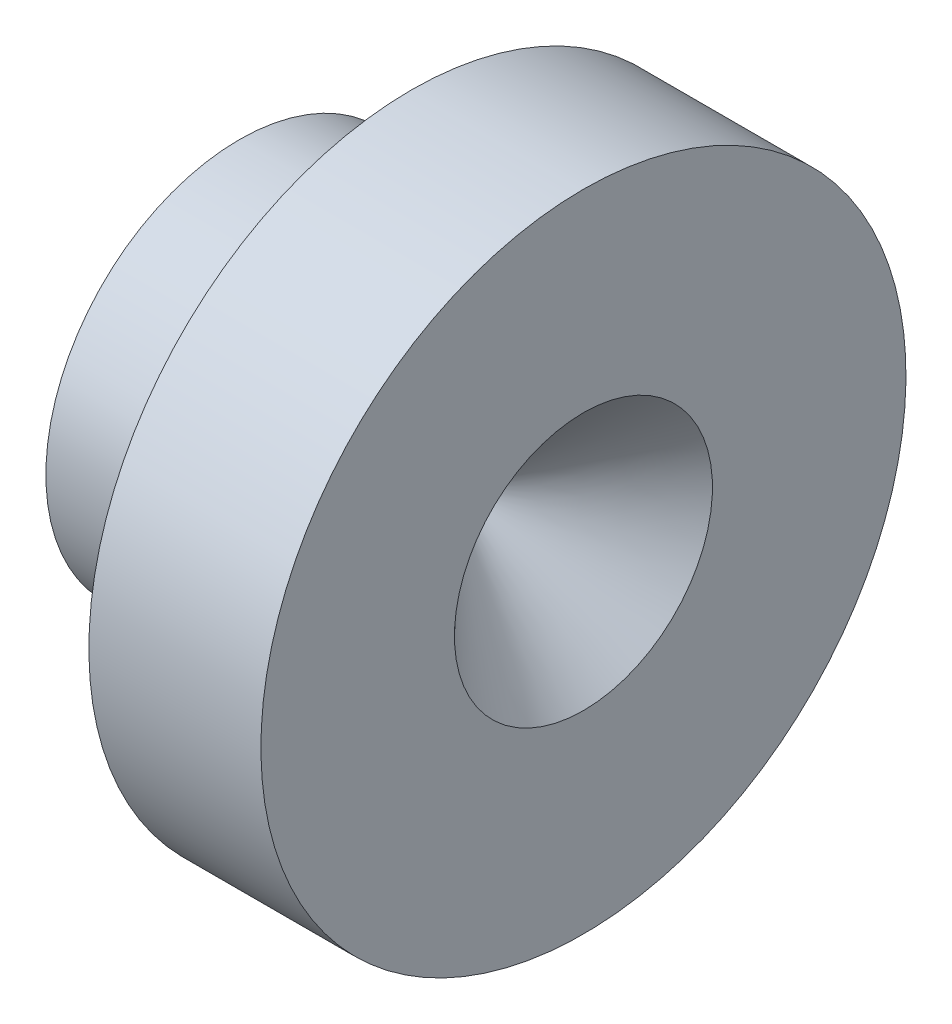
from build123d import *


with BuildPart() as part:
    # Sketch1 → Revolve1 (revolve)
    with BuildSketch(Plane.XY):
        Polygon((0, 4.5), (0, 0.5), (5.5, 0.5), (8, 3), (8, 7.5), (4, 7.5), (4, 4.5), align=None)
    revolve(axis=Axis((8, 0, 0), (-1, 0, 0)))


solid = part.part
